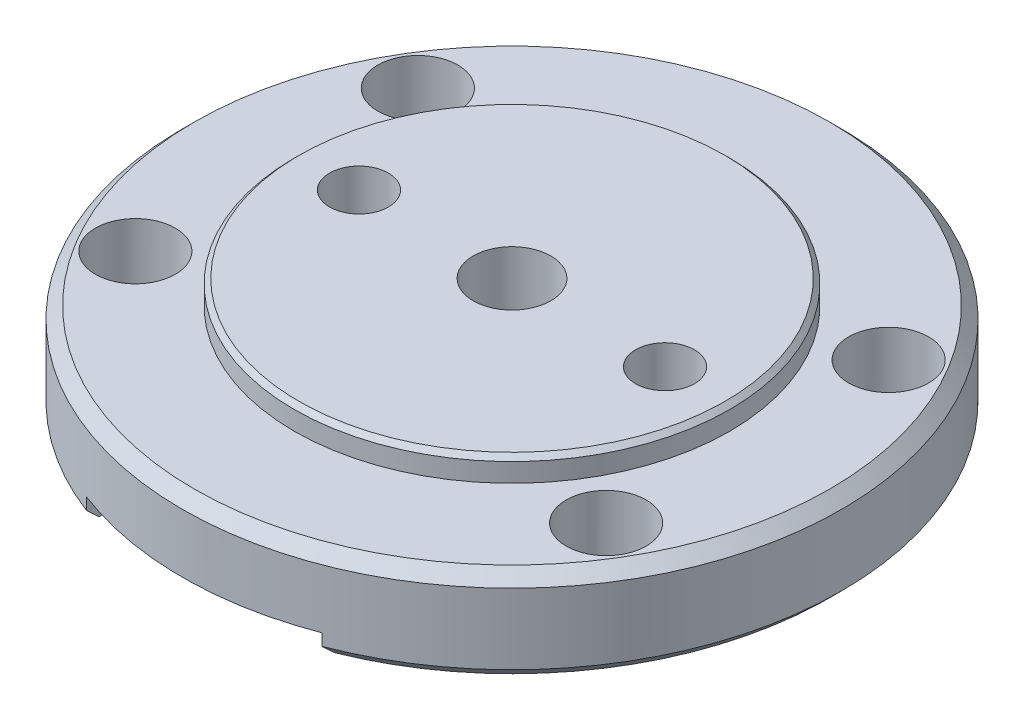
from build123d import *

# Parameters (mm, degrees)
M3_TAPPED_HOLE1_D    = 2.5
SKETCH3_OUTSIDE_W    = 37.982
SKETCH3_OUTSIDE_H    = 37.982
SKETCH3_OUTSIDE_R    = 9.25
CUT_EXTRUDE2_DEPTH   = 1
M3_CLEARANCE_HOLE1_D = 3.4
SKETCH6_W            = 10
SKETCH6_H            = 31.428384658
CUT_EXTRUDE3_DEPTH   = 1
M4_TAPPED_HOLE1_D    = 3.3
CHAMFER1_SIZE        = 0.5
CHAMFER2_SIZE        = 0.2


with BuildPart() as part:
    # Sketch1 → Revolve1 (revolve)
    with BuildSketch(Plane.XY, mode=Mode.PRIVATE) as revolve1_sk:
        Polygon((4.5, 5), (6, 5), (14, 5), (14, 0), (0, 0), (0, 5), align=None)
    revolve(revolve1_sk.sketch.rotate(Axis((0, 0, 0), (0, 1, 0)), 90), axis=Axis((0, 0, 0), (0, 1, 0)))

    # M3 Tapped Hole1 (through all)
    with Locations(Plane(origin=(0, 5, 0), x_dir=(1, 0, 0), z_dir=(0, 1, 0))):
        with Locations((-6.5, 0), (6.5, 0)):
            Hole(M3_TAPPED_HOLE1_D / 2)

    # Sketch3 outside → Cut-Extrude2 (cut)
    with BuildSketch(Plane(origin=(0, 5, 0), x_dir=(1, 0, 0), z_dir=(0, 1, 0))):
        Rectangle(SKETCH3_OUTSIDE_W, SKETCH3_OUTSIDE_H)
        with Locations(Location((0, 0, 0), (0, 0, 270))):
            Circle(SKETCH3_OUTSIDE_R, mode=Mode.SUBTRACT)
    extrude(amount=-CUT_EXTRUDE2_DEPTH, mode=Mode.SUBTRACT)

    # M3 Clearance Hole1 (through all)
    with Locations(Plane(origin=(0, 0, 0), x_dir=(-1, 0, 0), z_dir=(0, -1, 0))):
        with Locations((10, -6), (10, 6), (-10, -6), (-10, 6)):
            Hole(M3_CLEARANCE_HOLE1_D / 2)

    # Sketch6 → Cut-Extrude3 (cut)
    with BuildSketch(Plane.XZ):
        Rectangle(SKETCH6_W, SKETCH6_H)
    extrude(amount=-CUT_EXTRUDE3_DEPTH, mode=Mode.SUBTRACT)

    # M4 Tapped Hole1 (through all)
    with Locations(Plane(origin=(0, 1, 0), x_dir=(-1, 0, 0), z_dir=(0, -1, 0))):
        with Locations((0, 0)):
            Hole(M4_TAPPED_HOLE1_D / 2)

    # Chamfer1
    chamfer1_edges = [part.edges().sort_by_distance(p)[0] for p in [
        (0, 4, 14),
        (14, 0, 0),
        (-14, 0, 0),
    ]]
    chamfer(chamfer1_edges, length=CHAMFER1_SIZE)

    # Chamfer2
    chamfer2_edges = [part.edges().sort_by_distance(p)[0] for p in [
        (0, 5, -9.25),
    ]]
    chamfer(chamfer2_edges, length=CHAMFER2_SIZE)


solid = part.part
